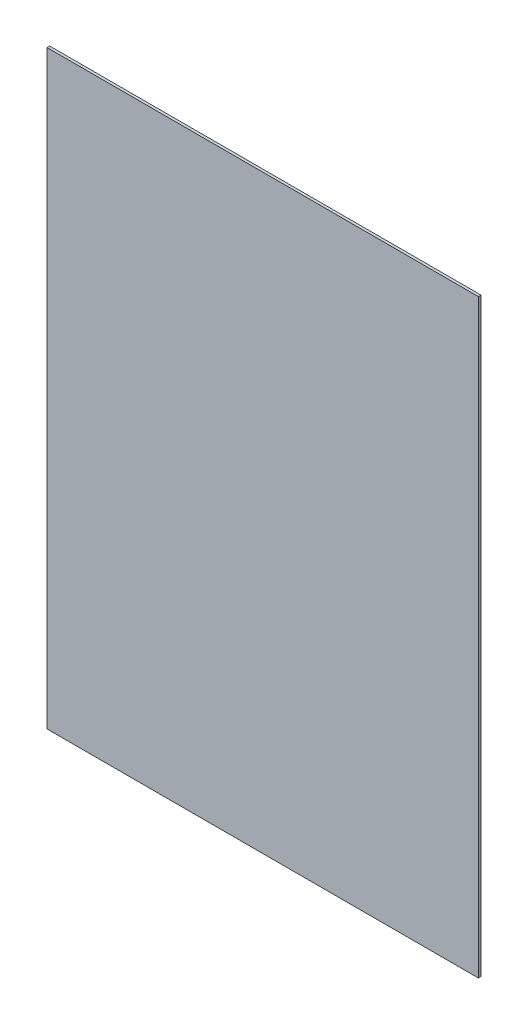
SolidWorks part; units mm, degrees
ref_plane "前视" through (0, 0, 0) normal (0, 0, 1) x (1, 0, 0)
ref_plane "上视" through (0, 0, 0) normal (0, 1, 0) x (1, 0, 0)
ref_plane "右视" through (0, 0, 0) normal (1, 0, 0) x (0, 0, -1)
sketch "草图1" plane through (0, 0, 0) normal (0, 0, 1) x (1, 0, 0)
  line L1 (-409, 559.5) -> (409, 559.5)
  line L2 (-409, 559.5) -> (-409, -559.5)
  line L3 (-409, -559.5) -> (409, -559.5)
  line L4 (409, 559.5) -> (409, -559.5)
  line L5 (-409, 559.5) -> (409, -559.5) construction
  line L6 (-409, -559.5) -> (409, 559.5) construction
  point P0 (0, 0)
  dimension "D1" = 1119
  dimension "D2" = 818
extrude "凸台-拉伸1" add sketch "草图1" along normal blind 5
